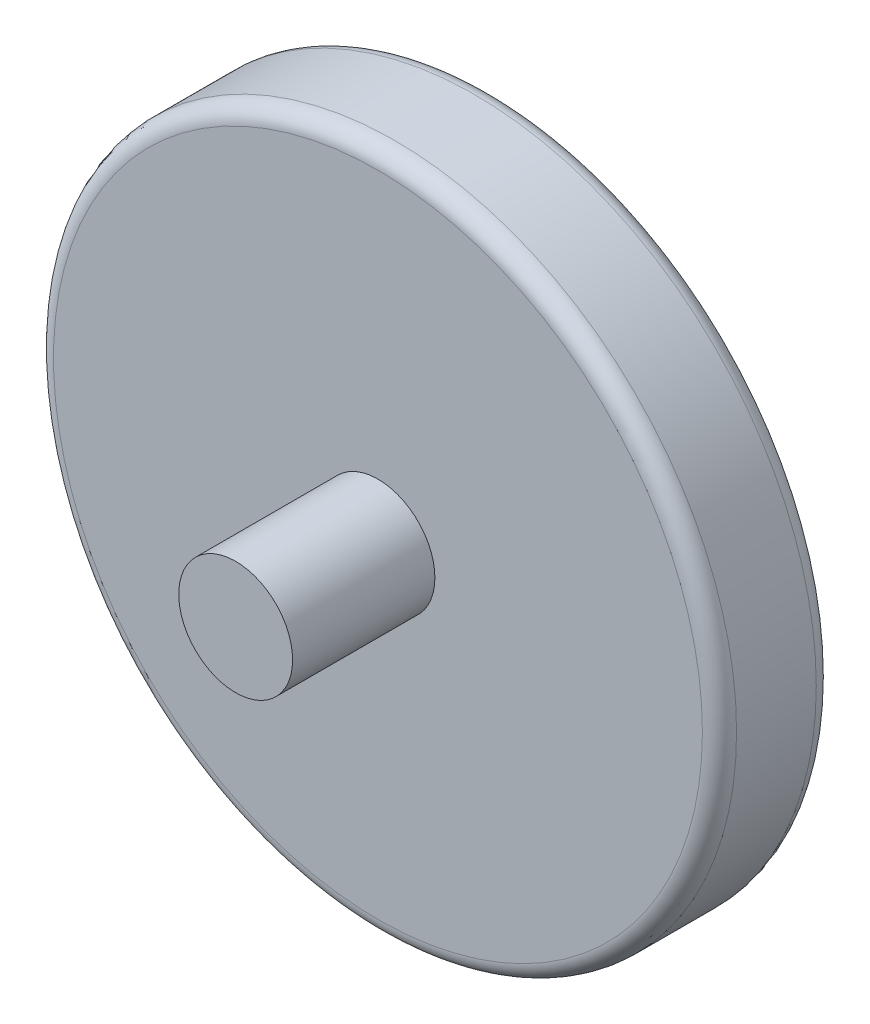
from build123d import *

# Parameters (mm, degrees)
SKETCH1_R           = 60
BOSS_EXTRUDE1_DEPTH = 20
FILLET1_R           = 3
SKETCH2_R           = 10
BOSS_EXTRUDE2_DEPTH = 25
BOSS_EXTRUDE3_START = 25
SKETCH3_R           = 10
BOSS_EXTRUDE3_DEPTH = 25


with BuildPart() as part:
    # Sketch1 → Boss-Extrude1 (new body)
    with BuildSketch(Plane.XY):
        Circle(SKETCH1_R)
    extrude(amount=BOSS_EXTRUDE1_DEPTH)

    # Fillet1
    fillet1_edges = [part.edges().sort_by_distance(p)[0] for p in [
        (-60, 0, 0),
        (-60, 0, 20),
    ]]
    fillet(fillet1_edges, radius=FILLET1_R)

    # Sketch2 → Boss-Extrude2 (add)
    with BuildSketch(Plane(origin=(0, 0, 0), x_dir=(-1, 0, 0), z_dir=(0, 0, -1))):
        with Locations(Location((0, 0, 0), (0, 0, 180))):
            Circle(SKETCH2_R)
    extrude(amount=BOSS_EXTRUDE2_DEPTH)

    # Sketch3 → Boss-Extrude3 (add)
    with BuildSketch(Plane.XY.offset(20).offset(BOSS_EXTRUDE3_START)):
        Circle(SKETCH3_R)
    extrude(amount=-BOSS_EXTRUDE3_DEPTH)


solid = part.part
